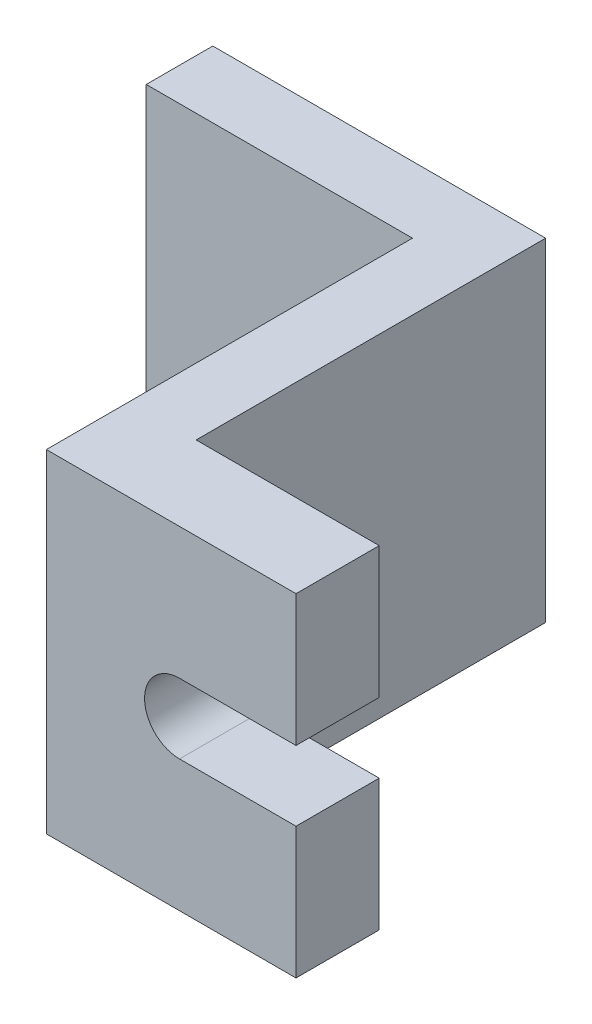
from build123d import *

# Parameters (mm, degrees)
SKETCH1_W           = 16
SKETCH1_H           = 4
SKETCH1_W_2         = 4
SKETCH1_H_2         = 17
SKETCH1_H_3         = 5
SKETCH1_W_3         = 11
BOSS_EXTRUDE1_DEPTH = 20
CUT_EXTRUDE1_DEPTH  = 15


with BuildPart() as part:
    # Sketch1 → Boss-Extrude1 (new body)
    with BuildSketch(Plane(origin=(0, 0, 0), x_dir=(1, 0, 0), z_dir=(0, 1, 0))):
        with Locations((-14.574257426, 6.653465347)):
            Rectangle(SKETCH1_W, SKETCH1_H)
        with Locations((-4.574257426, 6.653465347)):
            Rectangle(SKETCH1_W_2, SKETCH1_H)
        with Locations((-4.574257426, -3.846534653)):
            Rectangle(SKETCH1_W_2, SKETCH1_H_2)
        with Locations((-4.574257426, -14.846534653)):
            Rectangle(SKETCH1_W_2, SKETCH1_H_3)
        with Locations((2.925742574, -14.846534653)):
            Rectangle(SKETCH1_W_3, SKETCH1_H_3)
    extrude(amount=BOSS_EXTRUDE1_DEPTH)

    # Sketch2 → Cut-Extrude1 (cut)
    with BuildSketch(Plane(origin=(0, 0, 12.346534653), x_dir=(-1, 0, 0), z_dir=(0, 0, -1))):
        with BuildLine():
            Line((-5.425742574, 7.9), (-8.841676891, 7.9))
            Line((-8.841676891, 7.9), (-8.841676891, 11.852277474))
            Line((-8.841676891, 11.852277474), (-8.841676891, 12.1))
            Line((-8.841676891, 12.1), (-5.425742574, 12.1))
            Line((-5.425742574, 12.1), (-1.425742574, 12.1))
            ThreePointArc((-1.425742574, 12.1), (0.674257426, 10), (-1.425742574, 7.9))
            Line((-1.425742574, 7.9), (-5.425742574, 7.9))
        make_face()
    extrude(amount=-CUT_EXTRUDE1_DEPTH, mode=Mode.SUBTRACT)


solid = part.part
